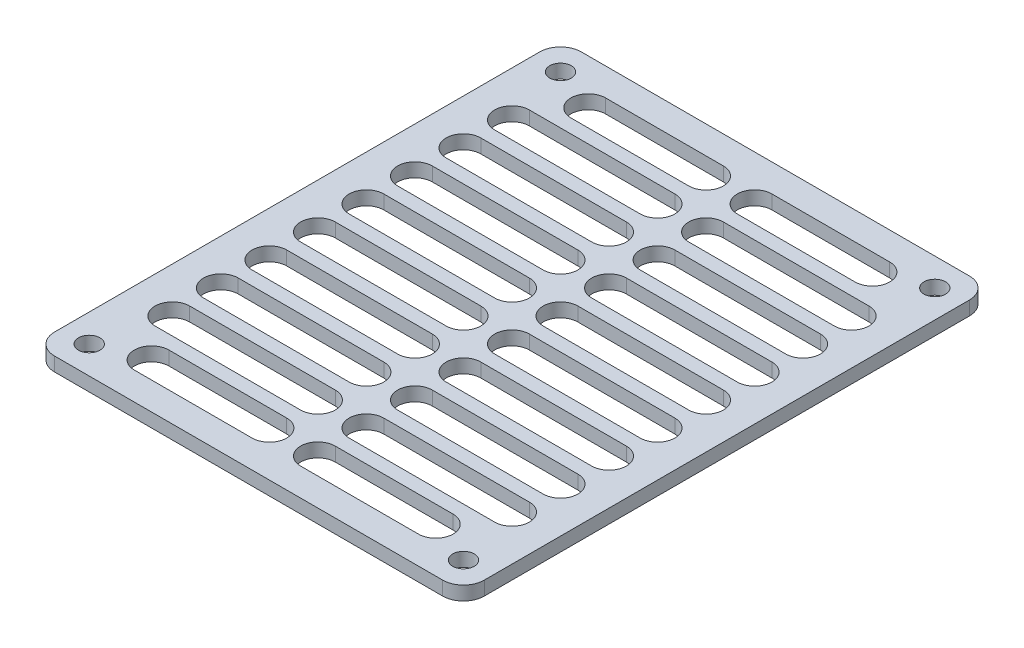
SolidWorks part; units mm, degrees
material "Thornel Mat VMA"
ref_plane "前视基准面" through (0, 0, 0) normal (0, 0, 1) x (1, 0, 0)
ref_plane "上视基准面" through (0, 0, 0) normal (0, 1, 0) x (1, 0, 0)
ref_plane "右视基准面" through (0, 0, 0) normal (1, 0, 0) x (0, 0, -1)
other "Configuration Table"
sketch "草图1" plane through (0, 0, 0) normal (0, 1, 0) x (1, 0, 0)
  line L0 (-31, 38) -> (-31, -38)
  line L1 (-27, 34) -> (27, 34) construction
  line L2 (-27, 34) -> (-27, -34) construction
  line L3 (-27, -34) -> (27, -34) construction
  line L4 (27, 34) -> (27, -34) construction
  line L5 (-27, 34) -> (27, -34) construction
  line L6 (-27, -34) -> (27, 34) construction
  line L7 (-31, -38) -> (31, -38)
  line L8 (31, 38) -> (31, -38)
  line L9 (-31, 38) -> (31, 38)
  line L10 (0, 0) -> (49.815, 0) construction
  line L11 (0, 0) -> (0, 60.3183) construction
  line L12 (3.5, 3.5) -> (20.5, 3.5) construction
  line L15 (3.5, 6) -> (20.5, 6)
  line L18 (3.5, 1) -> (20.5, 1)
  line L21 (-3.5, 3.5) -> (-20.5, 3.5) construction
  line L24 (-3.5, 6) -> (-20.5, 6)
  line L27 (-3.5, 1) -> (-20.5, 1)
  line L30 (3.5, 10.5) -> (20.5, 10.5) construction
  line L33 (3.5, 13) -> (20.5, 13)
  line L36 (3.5, 8) -> (20.5, 8)
  line L39 (-3.5, 10.5) -> (-20.5, 10.5) construction
  line L42 (-3.5, 13) -> (-20.5, 13)
  line L45 (-3.5, 8) -> (-20.5, 8)
  line L48 (3.5, 17.5) -> (20.5, 17.5) construction
  line L51 (3.5, 20) -> (20.5, 20)
  line L54 (3.5, 15) -> (20.5, 15)
  line L57 (-3.5, 17.5) -> (-20.5, 17.5) construction
  line L60 (-3.5, 20) -> (-20.5, 20)
  line L61 (-3.5, 15) -> (-20.5, 15)
  line L62 (3.5, 24.5) -> (20.5, 24.5) construction
  line L63 (3.5, 27) -> (20.5, 27)
  line L64 (3.5, 22) -> (20.5, 22)
  line L65 (-3.5, 24.5) -> (-20.5, 24.5) construction
  line L66 (-3.5, 27) -> (-20.5, 27)
  line L67 (-3.5, 22) -> (-20.5, 22)
  line L68 (3.5, 31.5) -> (20.5, 31.5) construction
  line L69 (3.5, 34) -> (20.5, 34)
  line L70 (3.5, 29) -> (20.5, 29)
  line L71 (-3.5, 31.5) -> (-20.5, 31.5) construction
  line L72 (-3.5, 34) -> (-20.5, 34)
  line L73 (-3.5, 29) -> (-20.5, 29)
  line L74 (-3.5, -31.5) -> (-20.5, -31.5) construction
  line L75 (-3.5, -34) -> (-20.5, -34)
  line L76 (-3.5, -29) -> (-20.5, -29)
  line L77 (3.5, -31.5) -> (20.5, -31.5) construction
  line L78 (3.5, -34) -> (20.5, -34)
  line L79 (3.5, -29) -> (20.5, -29)
  line L80 (-3.5, -24.5) -> (-20.5, -24.5) construction
  line L81 (-3.5, -27) -> (-20.5, -27)
  line L82 (-3.5, -22) -> (-20.5, -22)
  line L83 (3.5, -24.5) -> (20.5, -24.5) construction
  line L84 (3.5, -27) -> (20.5, -27)
  line L85 (3.5, -22) -> (20.5, -22)
  line L86 (-3.5, -17.5) -> (-20.5, -17.5) construction
  line L87 (-3.5, -20) -> (-20.5, -20)
  line L88 (-3.5, -15) -> (-20.5, -15)
  line L89 (3.5, -17.5) -> (20.5, -17.5) construction
  line L90 (3.5, -20) -> (20.5, -20)
  line L91 (3.5, -15) -> (20.5, -15)
  line L92 (-3.5, -10.5) -> (-20.5, -10.5) construction
  line L93 (-3.5, -13) -> (-20.5, -13)
  line L94 (-3.5, -8) -> (-20.5, -8)
  line L95 (3.5, -10.5) -> (20.5, -10.5) construction
  line L96 (3.5, -13) -> (20.5, -13)
  line L97 (3.5, -8) -> (20.5, -8)
  line L98 (-3.5, -3.5) -> (-20.5, -3.5) construction
  line L99 (-3.5, -6) -> (-20.5, -6)
  line L100 (-3.5, -1) -> (-20.5, -1)
  line L101 (3.5, -3.5) -> (20.5, -3.5) construction
  line L102 (3.5, -6) -> (20.5, -6)
  line L103 (3.5, -1) -> (20.5, -1)
  line L104 (20.5, 6) -> (24.5, 6)
  line L105 (20.5, 1) -> (24.5, 1)
  line L106 (-20.5, 1) -> (-24.5, 1)
  line L107 (-20.5, 6) -> (-24.5, 6)
  line L108 (20.5, 13) -> (24.5, 13)
  line L109 (20.5, 8) -> (24.5, 8)
  line L110 (-20.5, 13) -> (-24.5, 13)
  line L111 (-20.5, 8) -> (-24.5, 8)
  line L112 (20.5, 20) -> (24.5, 20)
  line L113 (20.5, 15) -> (24.5, 15)
  line L114 (-20.5, 20) -> (-24.5, 20)
  line L115 (-20.5, 15) -> (-24.5, 15)
  line L116 (20.5, 27) -> (24.5, 27)
  line L117 (20.5, 22) -> (24.5, 22)
  line L118 (-20.5, 27) -> (-24.5, 27)
  line L119 (-20.5, 22) -> (-24.5, 22)
  line L120 (20.5, -27) -> (24.5, -27)
  line L121 (20.5, -22) -> (24.5, -22)
  line L122 (20.5, -20) -> (24.5, -20)
  line L123 (20.5, -15) -> (24.5, -15)
  line L124 (20.5, -13) -> (24.5, -13)
  line L125 (20.5, -8) -> (24.5, -8)
  line L126 (20.5, -6) -> (24.5, -6)
  line L127 (20.5, -1) -> (24.5, -1)
  line L128 (-20.5, -1) -> (-24.5, -1)
  line L129 (-20.5, -6) -> (-24.5, -6)
  line L130 (-20.5, -8) -> (-24.5, -8)
  line L131 (-20.5, -13) -> (-24.5, -13)
  line L132 (-20.5, -15) -> (-24.5, -15)
  line L133 (-20.5, -20) -> (-24.5, -20)
  line L134 (-20.5, -22) -> (-24.5, -22)
  line L135 (-20.5, -27) -> (-24.5, -27)
  circle A0 centre (-27, 34) radius 1.55
  circle A1 centre (27, 34) radius 1.55
  circle A2 centre (27, -34) radius 1.55
  circle A3 centre (-27, -34) radius 1.55
  arc A36 (3.5, 6) -> (3.5, 1) centre (3.5, 3.5) ccw
  arc A37 (20.5, 1) -> (20.5, 6) centre (20.5, 3.5) ccw
  arc A38 (-3.5, 6) -> (-3.5, 1) centre (-3.5, 3.5) cw
  arc A39 (-20.5, 1) -> (-20.5, 6) centre (-20.5, 3.5) cw
  arc A40 (3.5, 13) -> (3.5, 8) centre (3.5, 10.5) ccw
  arc A41 (20.5, 8) -> (20.5, 13) centre (20.5, 10.5) ccw
  arc A42 (-3.5, 13) -> (-3.5, 8) centre (-3.5, 10.5) cw
  arc A43 (-20.5, 8) -> (-20.5, 13) centre (-20.5, 10.5) cw
  arc A44 (3.5, 20) -> (3.5, 15) centre (3.5, 17.5) ccw
  arc A45 (20.5, 15) -> (20.5, 20) centre (20.5, 17.5) ccw
  arc A46 (-3.5, 20) -> (-3.5, 15) centre (-3.5, 17.5) cw
  arc A47 (-20.5, 15) -> (-20.5, 20) centre (-20.5, 17.5) cw
  arc A48 (3.5, 27) -> (3.5, 22) centre (3.5, 24.5) ccw
  arc A49 (20.5, 22) -> (20.5, 27) centre (20.5, 24.5) ccw
  arc A50 (-3.5, 27) -> (-3.5, 22) centre (-3.5, 24.5) cw
  arc A51 (-20.5, 22) -> (-20.5, 27) centre (-20.5, 24.5) cw
  arc A52 (3.5, 34) -> (3.5, 29) centre (3.5, 31.5) ccw
  arc A53 (20.5, 29) -> (20.5, 34) centre (20.5, 31.5) ccw
  arc A54 (-3.5, 34) -> (-3.5, 29) centre (-3.5, 31.5) cw
  arc A55 (-20.5, 29) -> (-20.5, 34) centre (-20.5, 31.5) cw
  arc A56 (-3.5, -34) -> (-3.5, -29) centre (-3.5, -31.5) ccw
  arc A57 (-20.5, -29) -> (-20.5, -34) centre (-20.5, -31.5) ccw
  arc A58 (3.5, -34) -> (3.5, -29) centre (3.5, -31.5) cw
  arc A59 (20.5, -29) -> (20.5, -34) centre (20.5, -31.5) cw
  arc A60 (-3.5, -27) -> (-3.5, -22) centre (-3.5, -24.5) ccw
  arc A61 (-20.5, -22) -> (-20.5, -27) centre (-20.5, -24.5) ccw
  arc A62 (3.5, -27) -> (3.5, -22) centre (3.5, -24.5) cw
  arc A63 (20.5, -22) -> (20.5, -27) centre (20.5, -24.5) cw
  arc A64 (-3.5, -20) -> (-3.5, -15) centre (-3.5, -17.5) ccw
  arc A65 (-20.5, -15) -> (-20.5, -20) centre (-20.5, -17.5) ccw
  arc A66 (3.5, -20) -> (3.5, -15) centre (3.5, -17.5) cw
  arc A67 (20.5, -15) -> (20.5, -20) centre (20.5, -17.5) cw
  arc A68 (-3.5, -13) -> (-3.5, -8) centre (-3.5, -10.5) ccw
  arc A69 (-20.5, -8) -> (-20.5, -13) centre (-20.5, -10.5) ccw
  arc A70 (3.5, -13) -> (3.5, -8) centre (3.5, -10.5) cw
  arc A71 (20.5, -8) -> (20.5, -13) centre (20.5, -10.5) cw
  arc A72 (-3.5, -6) -> (-3.5, -1) centre (-3.5, -3.5) ccw
  arc A73 (-20.5, -1) -> (-20.5, -6) centre (-20.5, -3.5) ccw
  arc A74 (3.5, -6) -> (3.5, -1) centre (3.5, -3.5) cw
  arc A75 (20.5, -1) -> (20.5, -6) centre (20.5, -3.5) cw
  arc A76 (24.5, 6) -> (24.5, 1) centre (24.5, 3.5) cw
  arc A77 (-24.5, 6) -> (-24.5, 1) centre (-24.5, 3.5) ccw
  arc A78 (24.5, 13) -> (24.5, 8) centre (24.5, 10.5) cw
  arc A79 (-24.5, 13) -> (-24.5, 8) centre (-24.5, 10.5) ccw
  arc A80 (24.5, 20) -> (24.5, 15) centre (24.5, 17.5) cw
  arc A81 (-24.5, 20) -> (-24.5, 15) centre (-24.5, 17.5) ccw
  arc A82 (24.5, 27) -> (24.5, 22) centre (24.5, 24.5) cw
  arc A83 (-24.5, 27) -> (-24.5, 22) centre (-24.5, 24.5) ccw
  arc A84 (24.5, -27) -> (24.5, -22) centre (24.5, -24.5) ccw
  arc A85 (24.5, -20) -> (24.5, -15) centre (24.5, -17.5) ccw
  arc A86 (24.5, -13) -> (24.5, -8) centre (24.5, -10.5) ccw
  arc A87 (24.5, -6) -> (24.5, -1) centre (24.5, -3.5) ccw
  arc A88 (-24.5, -6) -> (-24.5, -1) centre (-24.5, -3.5) cw
  arc A89 (-24.5, -13) -> (-24.5, -8) centre (-24.5, -10.5) cw
  arc A90 (-24.5, -20) -> (-24.5, -15) centre (-24.5, -17.5) cw
  arc A91 (-24.5, -27) -> (-24.5, -22) centre (-24.5, -24.5) cw
  point P0 (0, 0)
  point P19 (12, 3.5)
  point P26 (-12, 3.5)
  point P34 (12, 10.5)
  point P41 (-12, 10.5)
  point P48 (12, 17.5)
  point P55 (-12, 17.5)
  point P62 (12, 24.5)
  point P69 (-12, 24.5)
  point P76 (12, 31.5)
  point P83 (-12, 31.5)
  point P89 (-12, -31.5)
  point P96 (12, -31.5)
  point P103 (-12, -24.5)
  point P110 (12, -24.5)
  point P117 (-12, -17.5)
  point P124 (12, -17.5)
  point P131 (-12, -10.5)
  point P138 (12, -10.5)
  point P145 (-12, -3.5)
  point P152 (12, -3.5)
  dimension "D3" = 3.1
  dimension "D7" = 12
  dimension "D6" = 2.5
  dimension "D1" = 68
  dimension "D2" = 54
  dimension "D5" = 1
  dimension "D8" = 17
  dimension "D10" = 2
  dimension "D4" = 4
  dimension "D9" = 5
  dimension "D11" = 4
extrude "凸台-拉伸1" add sketch "草图1" along normal blind 2 contours L9 L0 L7 L8 A73 L100 A72 L99 A69 L94 A68 L93 A65 L88 A64 L87 A61 L82 A60 L81 A57 L76 A56 L75 A53 L70 A52 L69 A49 L64 A48 L63 A41 L36 A40 L33 A37 L18 A36 L15 A3
fillet "圆角1" radius 3 4 edges at (31, 1, -38) (31, 1, 38) (-31, 1, 38) (-31, 1, -38)
